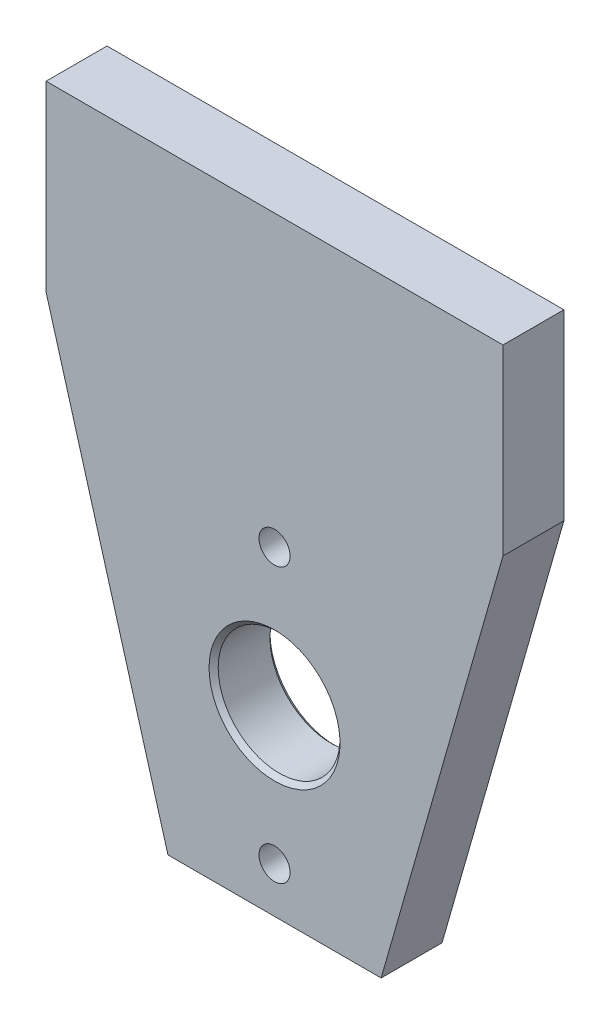
from build123d import *

# Parameters (mm, degrees)
SKETCH1_R              = 20
BOSS_EXTRUDE1_DEPTH    = 20
M12_TAPPED_HOLE1_D     = 10.2
M12_TAPPED_HOLE1_DEPTH = 29.25
M12_TAPPED_HOLE1_TIP   = 3.064389157
CHAMFER1_SIZE          = 1.5


with BuildPart() as part:
    # Sketch1 → Boss-Extrude1 (new body)
    with BuildSketch(Plane.XY):
        Polygon((0, 0), (150, 0), (150, -60), (110, -200), (40, -200), (0, -60), align=None)
        with Locations((75, -140)):
            Circle(SKETCH1_R, mode=Mode.SUBTRACT)
    extrude(amount=BOSS_EXTRUDE1_DEPTH)

    # M12 Tapped Hole1
    with Locations(Plane.XY.offset(20)):
        with Locations((75, -95), (75, -185)):
            Hole(M12_TAPPED_HOLE1_D / 2, depth=M12_TAPPED_HOLE1_DEPTH)
            with Locations((0, 0, -(M12_TAPPED_HOLE1_DEPTH + M12_TAPPED_HOLE1_TIP / 2))):  # 118° drill point
                Cone(0, M12_TAPPED_HOLE1_D / 2, M12_TAPPED_HOLE1_TIP, mode=Mode.SUBTRACT)

    # Chamfer1
    chamfer1_edges = [part.edges().sort_by_distance(p)[0] for p in [
        (55, -140, 0),
        (55, -140, 20),
    ]]
    chamfer(chamfer1_edges, length=CHAMFER1_SIZE)


solid = part.part
